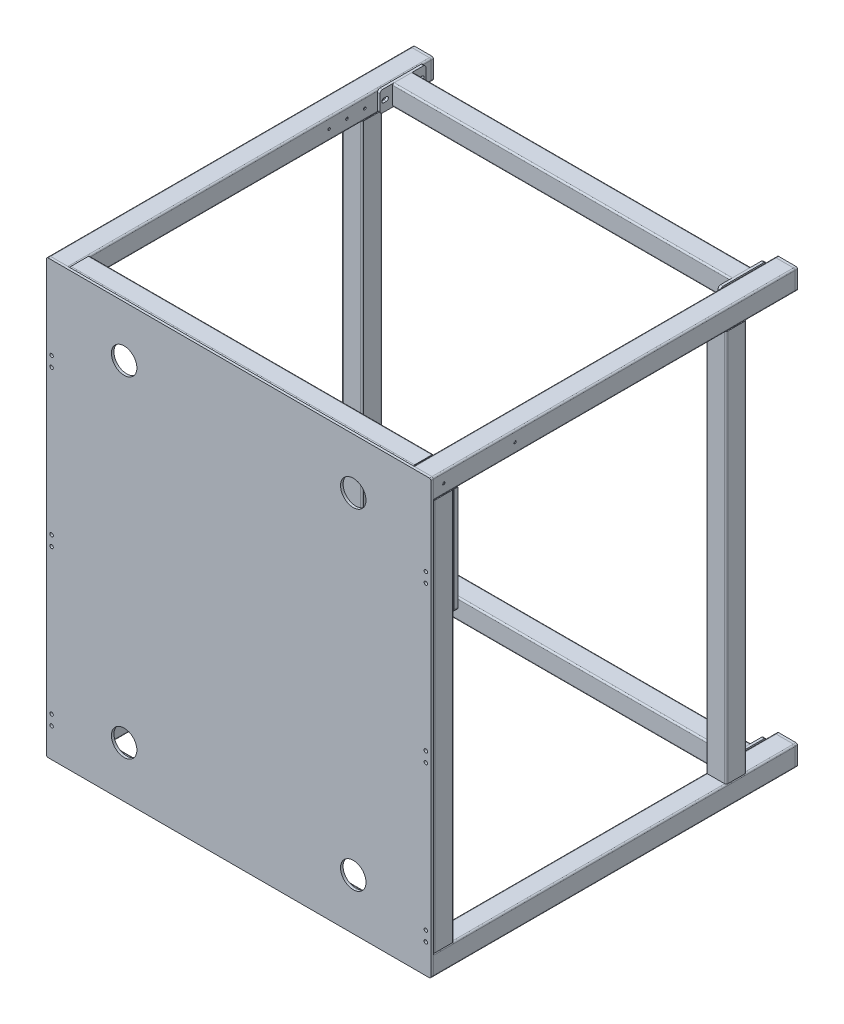
SolidWorks part; units mm, degrees
ref_plane "前视基准面" through (0, 0, 0) normal (0, 0, 1) x (1, 0, 0)
ref_plane "上视基准面" through (0, 0, 0) normal (0, 1, 0) x (1, 0, 0)
ref_plane "右视基准面" through (0, 0, 0) normal (1, 0, 0) x (0, 0, -1)
sketch "草图1" plane through (0, 0, 0) normal (0, 0, 1) x (1, 0, 0)
  line L1 (-377.5, 425) -> (377.5, 425)
  line L2 (-377.5, 425) -> (-377.5, -425)
  line L3 (-377.5, -425) -> (377.5, -425)
  line L4 (377.5, 425) -> (377.5, -425)
  line L5 (-377.5, 425) -> (377.5, -425) construction
  line L6 (-377.5, -425) -> (377.5, 425) construction
  point P0 (0, 0)
  dimension "D1" = 850
  dimension "D2" = 755
extrude "凸台-拉伸1" add sketch "草图1" along normal blind 5
sketch "草图3" plane through (0, 0, 0) normal (0, 0, -1) x (-1, 0, 0)
  line L0 (-377.5, -425) -> (-377.5, 425) construction
  line L1 (-377.5, 425) -> (377.5, 425) construction
  line L2 (377.5, 425) -> (377.5, -425) construction
  line L3 (377.5, -425) -> (-377.5, -425) construction
  line B0 (339.5, 388) -> (339.5, 422)
  line B1 (374.5, 385) -> (340.5, 385)
  line B2 (377.5, 388) -> (377.5, 422)
  line B3 (374.5, 425) -> (340.5, 425)
  line B4 (337.5, 388) -> (337.5, 422)
  line B5 (374.5, 423) -> (340.5, 423)
  line B6 (375.5, 388) -> (375.5, 422)
  line B7 (374.5, 387) -> (340.5, 387)
  arc B8 (377.5, 422) -> (374.5, 425) centre (374.5, 422) ccw
  arc B9 (374.5, 385) -> (377.5, 388) centre (374.5, 388) ccw
  arc B10 (340.5, 385) -> (337.5, 388) centre (340.5, 388) cw
  arc B11 (340.5, 425) -> (337.5, 422) centre (340.5, 422) ccw
  arc B12 (340.5, 423) -> (339.5, 422) centre (340.5, 422) ccw
  arc B13 (375.5, 422) -> (374.5, 423) centre (374.5, 422) ccw
  arc B14 (374.5, 387) -> (375.5, 388) centre (374.5, 388) ccw
  arc B15 (340.5, 387) -> (339.5, 388) centre (340.5, 388) cw
  line B16 (339.5, -422) -> (339.5, -388)
  line B17 (374.5, -425) -> (340.5, -425)
  line B18 (377.5, -422) -> (377.5, -388)
  line B19 (374.5, -385) -> (340.5, -385)
  line B20 (337.5, -422) -> (337.5, -388)
  line B21 (374.5, -387) -> (340.5, -387)
  line B22 (375.5, -422) -> (375.5, -388)
  line B23 (374.5, -423) -> (340.5, -423)
  arc B24 (377.5, -388) -> (374.5, -385) centre (374.5, -388) ccw
  arc B25 (374.5, -425) -> (377.5, -422) centre (374.5, -422) ccw
  arc B26 (340.5, -425) -> (337.5, -422) centre (340.5, -422) cw
  arc B27 (340.5, -385) -> (337.5, -388) centre (340.5, -388) ccw
  arc B28 (340.5, -387) -> (339.5, -388) centre (340.5, -388) ccw
  arc B29 (375.5, -388) -> (374.5, -387) centre (374.5, -388) ccw
  arc B30 (374.5, -423) -> (375.5, -422) centre (374.5, -422) ccw
  arc B31 (340.5, -423) -> (339.5, -422) centre (340.5, -422) cw
  line B32 (-375.5, -422) -> (-375.5, -388)
  line B33 (-340.5, -425) -> (-374.5, -425)
  line B34 (-337.5, -422) -> (-337.5, -388)
  line B35 (-340.5, -385) -> (-374.5, -385)
  line B36 (-377.5, -422) -> (-377.5, -388)
  line B37 (-340.5, -387) -> (-374.5, -387)
  line B38 (-339.5, -422) -> (-339.5, -388)
  line B39 (-340.5, -423) -> (-374.5, -423)
  arc B40 (-337.5, -388) -> (-340.5, -385) centre (-340.5, -388) ccw
  arc B41 (-340.5, -425) -> (-337.5, -422) centre (-340.5, -422) ccw
  arc B42 (-374.5, -425) -> (-377.5, -422) centre (-374.5, -422) cw
  arc B43 (-374.5, -385) -> (-377.5, -388) centre (-374.5, -388) ccw
  arc B44 (-374.5, -387) -> (-375.5, -388) centre (-374.5, -388) ccw
  arc B45 (-339.5, -388) -> (-340.5, -387) centre (-340.5, -388) ccw
  arc B46 (-340.5, -423) -> (-339.5, -422) centre (-340.5, -422) ccw
  arc B47 (-374.5, -423) -> (-375.5, -422) centre (-374.5, -422) cw
  line B48 (-375.5, 388) -> (-375.5, 422)
  line B49 (-340.5, 385) -> (-374.5, 385)
  line B50 (-337.5, 388) -> (-337.5, 422)
  line B51 (-340.5, 425) -> (-374.5, 425)
  line B52 (-377.5, 388) -> (-377.5, 422)
  line B53 (-340.5, 423) -> (-374.5, 423)
  line B54 (-339.5, 388) -> (-339.5, 422)
  line B55 (-340.5, 387) -> (-374.5, 387)
  arc B56 (-337.5, 422) -> (-340.5, 425) centre (-340.5, 422) ccw
  arc B57 (-340.5, 385) -> (-337.5, 388) centre (-340.5, 388) ccw
  arc B58 (-374.5, 385) -> (-377.5, 388) centre (-374.5, 388) cw
  arc B59 (-374.5, 425) -> (-377.5, 422) centre (-374.5, 422) ccw
  arc B60 (-374.5, 423) -> (-375.5, 422) centre (-374.5, 422) ccw
  arc B61 (-339.5, 422) -> (-340.5, 423) centre (-340.5, 422) ccw
  arc B62 (-340.5, 387) -> (-339.5, 388) centre (-340.5, 388) ccw
  arc B63 (-374.5, 387) -> (-375.5, 388) centre (-374.5, 388) cw
sketch_block_instance "方管4040-1"
sketch_block "方管4040" parameters "D2"=3, "D1"=40
sketch_block_instance "方管4040-2"
sketch_block_instance "方管4040-3"
sketch_block_instance "方管4040-4"
extrude "凸台-拉伸3" add sketch "草图3" along normal blind 710 separate body
fillet "圆角1" radius 3 4 edges at (377.5, 425, 2.5) (377.5, -425, 2.5) (-377.5, -425, 2.5) (-377.5, 425, 2.5)
sketch "草图4" plane through (-337.5, 0, 0) normal (1, 0, 0) x (0, 0, -1)
  line L0 (710, -385) -> (0, -385) construction
  line L1 (0, -388) -> (0, -422) construction
  line L2 (0, 422) -> (0, 388) construction
  line L3 (710, 425) -> (0, 425) construction
  line B0 (2, 388) -> (2, 422)
  line B1 (37, 385) -> (3, 385)
  line B2 (40, 388) -> (40, 422)
  line B3 (37, 425) -> (3, 425)
  line B4 (0, 388) -> (0, 422)
  line B5 (37, 423) -> (3, 423)
  line B6 (38, 388) -> (38, 422)
  line B7 (37, 387) -> (3, 387)
  arc B8 (40, 422) -> (37, 425) centre (37, 422) ccw
  arc B9 (37, 385) -> (40, 388) centre (37, 388) ccw
  arc B10 (3, 385) -> (0, 388) centre (3, 388) cw
  arc B11 (3, 425) -> (0, 422) centre (3, 422) ccw
  arc B12 (3, 423) -> (2, 422) centre (3, 422) ccw
  arc B13 (38, 422) -> (37, 423) centre (37, 422) ccw
  arc B14 (37, 387) -> (38, 388) centre (37, 388) ccw
  arc B15 (3, 387) -> (2, 388) centre (3, 388) cw
  line B16 (2, -422) -> (2, -388)
  line B17 (37, -425) -> (3, -425)
  line B18 (40, -422) -> (40, -388)
  line B19 (37, -385) -> (3, -385)
  line B20 (0, -422) -> (0, -388)
  line B21 (37, -387) -> (3, -387)
  line B22 (38, -422) -> (38, -388)
  line B23 (37, -423) -> (3, -423)
  arc B24 (40, -388) -> (37, -385) centre (37, -388) ccw
  arc B25 (37, -425) -> (40, -422) centre (37, -422) ccw
  arc B26 (3, -425) -> (0, -422) centre (3, -422) cw
  arc B27 (3, -385) -> (0, -388) centre (3, -388) ccw
  arc B28 (3, -387) -> (2, -388) centre (3, -388) ccw
  arc B29 (38, -388) -> (37, -387) centre (37, -388) ccw
  arc B30 (37, -423) -> (38, -422) centre (37, -422) ccw
  arc B31 (3, -423) -> (2, -422) centre (3, -422) cw
sketch_block_instance "方管4040-6"
sketch_block_instance "方管4040-8"
extrude "凸台-拉伸4" add sketch "草图4" along normal up to surface (675 mm away) separate body up to face at (337.5, 405, -355)
sketch "草图5" plane through (0, -385, 0) normal (0, 1, 0) x (1, 0, 0)
  line L0 (-377.5, 710) -> (-377.5, 0) construction
  line L1 (-374.5, 0) -> (-340.5, 0) construction
  line L2 (377.5, 710) -> (377.5, 0) construction
  line L3 (340.5, 0) -> (374.5, 0) construction
  line B0 (339.5, 3) -> (339.5, 37)
  line B1 (374.5, 0) -> (340.5, 0)
  line B2 (377.5, 3) -> (377.5, 37)
  line B3 (374.5, 40) -> (340.5, 40)
  line B4 (337.5, 3) -> (337.5, 37)
  line B5 (374.5, 38) -> (340.5, 38)
  line B6 (375.5, 3) -> (375.5, 37)
  line B7 (374.5, 2) -> (340.5, 2)
  arc B8 (377.5, 37) -> (374.5, 40) centre (374.5, 37) ccw
  arc B9 (374.5, 0) -> (377.5, 3) centre (374.5, 3) ccw
  arc B10 (340.5, 0) -> (337.5, 3) centre (340.5, 3) cw
  arc B11 (340.5, 40) -> (337.5, 37) centre (340.5, 37) ccw
  arc B12 (340.5, 38) -> (339.5, 37) centre (340.5, 37) ccw
  arc B13 (375.5, 37) -> (374.5, 38) centre (374.5, 37) ccw
  arc B14 (374.5, 2) -> (375.5, 3) centre (374.5, 3) ccw
  arc B15 (340.5, 2) -> (339.5, 3) centre (340.5, 3) cw
  line B16 (-375.5, 3) -> (-375.5, 37)
  line B17 (-340.5, 0) -> (-374.5, 0)
  line B18 (-337.5, 3) -> (-337.5, 37)
  line B19 (-340.5, 40) -> (-374.5, 40)
  line B20 (-377.5, 3) -> (-377.5, 37)
  line B21 (-340.5, 38) -> (-374.5, 38)
  line B22 (-339.5, 3) -> (-339.5, 37)
  line B23 (-340.5, 2) -> (-374.5, 2)
  arc B24 (-337.5, 37) -> (-340.5, 40) centre (-340.5, 37) ccw
  arc B25 (-340.5, 0) -> (-337.5, 3) centre (-340.5, 3) ccw
  arc B26 (-374.5, 0) -> (-377.5, 3) centre (-374.5, 3) cw
  arc B27 (-374.5, 40) -> (-377.5, 37) centre (-374.5, 37) ccw
  arc B28 (-374.5, 38) -> (-375.5, 37) centre (-374.5, 37) ccw
  arc B29 (-339.5, 37) -> (-340.5, 38) centre (-340.5, 37) ccw
  arc B30 (-340.5, 2) -> (-339.5, 3) centre (-340.5, 3) ccw
  arc B31 (-374.5, 2) -> (-375.5, 3) centre (-374.5, 3) cw
sketch_block_instance "方管4040-10"
sketch_block_instance "方管4040-11"
extrude "凸台-拉伸5" add sketch "草图5" along normal up to surface (770 mm away) separate body up to face at (-357.5, 385, -355)
sketch "草图6" plane through (0, 0, 5) normal (0, 0, 1) x (1, 0, 0)
  line L0 (367.5, 262.5) -> (367.5, -367.5) construction
  line L1 (367.5, 262.5) -> (-367.5, 262.5) construction
  line L2 (367.5, 262.5) -> (367.5, -367.5) construction
  line L3 (367.5, -367.5) -> (-367.5, -367.5) construction
  line L4 (-367.5, 262.5) -> (-367.5, -367.5) construction
  line L5 (367.5, 262.5) -> (-367.5, -367.5) construction
  line L6 (367.5, -367.5) -> (-367.5, 262.5) construction
  line L7 (0, -425) -> (0, -367.5) construction
  line L8 (-374.5, -425) -> (374.5, -425) construction
  circle A0 centre (-367.5, -367.5) radius 3.4
  circle A1 centre (367.5, -367.5) radius 3.4 construction
  circle A2 centre (367.5, 262.5) radius 3.4 construction
  circle A3 centre (-367.5, 262.5) radius 3.4 construction
  circle A4 centre (-367.5, -347.5) radius 3.4
  circle A5 centre (367.5, 262.5) radius 3.4 construction
  circle A6 centre (367.5, 262.5) radius 3.4
  circle A7 centre (-367.5, -62.5) radius 3.4
  circle A8 centre (-367.5, -42.5) radius 3.4
  circle A9 centre (-367.5, 242.5) radius 3.4
  circle A10 centre (-367.5, 262.5) radius 3.4
  circle A11 centre (367.5, 242.5) radius 3.4
  circle A12 centre (367.5, -42.5) radius 3.4
  circle A13 centre (367.5, -62.5) radius 3.4
  circle A14 centre (367.5, -347.5) radius 3.4
  circle A15 centre (367.5, -367.5) radius 3.4
  dimension "D3" = 6.8
  dimension "D5" = 20
  dimension "D6" = 3
  dimension "D1" = 735
  dimension "D2" = 630
  dimension "D4" = 57.5
extrude "切除-拉伸1" cut sketch "草图6" against normal blind 30
sketch "草图7" plane through (0, 0, -710) normal (0, 0, -1) x (-1, 0, 0)
  line L0 (-340.5, 425) -> (-374.5, 425) construction
  line L1 (-377.5, 422) -> (-377.5, 388) construction
  line L2 (377.5, 388) -> (377.5, 422) construction
  line L3 (374.5, 425) -> (340.5, 425) construction
  line L4 (374.5, -385) -> (340.5, -385) construction
  line L5 (377.5, -422) -> (377.5, -388) construction
  line B0 (337.5, 422) -> (337.5, 388)
  line B1 (340.5, 385) -> (374.5, 385)
  line B2 (377.5, 388) -> (377.5, 422)
  line B3 (374.5, 425) -> (340.5, 425)
  circle B4 centre (357.5, 405) radius 9.5
  arc B5 (340.5, 425) -> (337.5, 422) centre (340.5, 422) ccw
  arc B6 (337.5, 388) -> (340.5, 385) centre (340.5, 388) ccw
  arc B7 (374.5, 385) -> (377.5, 388) centre (374.5, 388) ccw
  arc B8 (377.5, 422) -> (374.5, 425) centre (374.5, 422) ccw
  line B9 (337.5, -388) -> (337.5, -422)
  line B10 (340.5, -425) -> (374.5, -425)
  line B11 (377.5, -422) -> (377.5, -388)
  line B12 (374.5, -385) -> (340.5, -385)
  circle B13 centre (357.5, -405) radius 9.5
  arc B14 (340.5, -385) -> (337.5, -388) centre (340.5, -388) ccw
  arc B15 (337.5, -422) -> (340.5, -425) centre (340.5, -422) ccw
  arc B16 (374.5, -425) -> (377.5, -422) centre (374.5, -422) ccw
  arc B17 (377.5, -388) -> (374.5, -385) centre (374.5, -388) ccw
  line B18 (-377.432, -388) -> (-377.432, -422)
  line B19 (-374.432, -425) -> (-340.432, -425)
  line B20 (-337.432, -422) -> (-337.432, -388)
  line B21 (-340.432, -385) -> (-374.432, -385)
  circle B22 centre (-357.432, -405) radius 9.5
  arc B23 (-374.432, -385) -> (-377.432, -388) centre (-374.432, -388) ccw
  arc B24 (-377.432, -422) -> (-374.432, -425) centre (-374.432, -422) ccw
  arc B25 (-340.432, -425) -> (-337.432, -422) centre (-340.432, -422) ccw
  arc B26 (-337.432, -388) -> (-340.432, -385) centre (-340.432, -388) ccw
  line B27 (-377.5, 422) -> (-377.5, 388)
  line B28 (-374.5, 385) -> (-340.5, 385)
  line B29 (-337.5, 388) -> (-337.5, 422)
  line B30 (-340.5, 425) -> (-374.5, 425)
  circle B31 centre (-357.5, 405) radius 9.5
  arc B32 (-374.5, 425) -> (-377.5, 422) centre (-374.5, 422) ccw
  arc B33 (-377.5, 388) -> (-374.5, 385) centre (-374.5, 388) ccw
  arc B34 (-340.5, 385) -> (-337.5, 388) centre (-340.5, 388) ccw
  arc B35 (-337.5, 422) -> (-340.5, 425) centre (-340.5, 422) ccw
sketch_block_instance "方管4040-M16-1"
sketch_block "方管4040-M16" parameters "D1"=19
sketch_block_instance "方管4040-M16-2"
sketch_block_instance "方管4040-M16-3"
sketch_block_instance "方管4040-M16-4"
extrude "凸台-拉伸6" add sketch "草图7" along normal blind 5 separate body
sketch "草图8" plane through (0, 0, -40) normal (0, 0, -1) x (-1, 0, 0)
  line L0 (-377.5, 385) -> (-377.5, -385) construction
  line L1 (-377.5, 175) -> (-317.5, 175)
  line L2 (-377.5, 175) -> (-377.5, 385)
  line L3 (-377.5, 385) -> (-317.5, 385)
  line L4 (-317.5, 175) -> (-317.5, 385)
  line L5 (-374.5, 385) -> (-340.5, 385) construction
  dimension "D1" = 60
  dimension "D2" = 210
extrude "凸台-拉伸7" add sketch "草图8" along normal blind 8 separate body
sketch "草图9" plane through (0, 0, -48) normal (0, 0, -1) x (-1, 0, 0)
  line L0 (-377.5, 280) -> (-317.5, 280) construction
  line L1 (-377.5, 385) -> (-377.5, 175) construction
  line L2 (-317.5, 175) -> (-317.5, 385) construction
  line L4 (-366.5, 187.5) -> (-328.5, 187.5) construction
  line L5 (-366.5, 187.5) -> (-366.5, 352.5) construction
  line L6 (-366.5, 352.5) -> (-328.5, 352.5) construction
  line L7 (-328.5, 187.5) -> (-328.5, 352.5) construction
  line L8 (-366.5, 187.5) -> (-328.5, 352.5) construction
  line L9 (-366.5, 352.5) -> (-328.5, 187.5) construction
  line L10 (-377.5, 175) -> (-317.5, 175) construction
  circle A0 centre (-366.5, 187.5) radius 3.4
  circle A1 centre (-328.5, 187.5) radius 3.4
  circle A2 centre (-366.5, 352.5) radius 3.4
  circle A3 centre (-328.5, 352.5) radius 3.4
  point P6 (-347.5, 270)
  dimension "D3" = 6.8
  dimension "D1" = 165
  dimension "D2" = 11
  dimension "D4" = 12.5
  dimension "D5" = 38
extrude "切除-拉伸2" cut sketch "草图9" against normal blind 10
fillet "圆角2" radius 5 3 edges at (317.5, 385, -44) (317.5, 175, -44) (377.5, 175, -44)
sketch "草图10" plane through (0, 385, 0) normal (0, -1, 0) x (1, 0, 0)
  line L0 (-377.5, -710) -> (-377.5, 0) construction
  line L1 (-340.5, -715) -> (-374.5, -715) construction
  line L2 (337.5, -710) -> (337.5, 0) construction
  line B0 (-375.5, -612) -> (-375.5, -578)
  line B1 (-340.5, -615) -> (-374.5, -615)
  line B2 (-337.5, -612) -> (-337.5, -578)
  line B3 (-340.5, -575) -> (-374.5, -575)
  line B4 (-377.5, -612) -> (-377.5, -578)
  line B5 (-340.5, -577) -> (-374.5, -577)
  line B6 (-339.5, -612) -> (-339.5, -578)
  line B7 (-340.5, -613) -> (-374.5, -613)
  arc B8 (-337.5, -578) -> (-340.5, -575) centre (-340.5, -578) ccw
  arc B9 (-340.5, -615) -> (-337.5, -612) centre (-340.5, -612) ccw
  arc B10 (-374.5, -615) -> (-377.5, -612) centre (-374.5, -612) cw
  arc B11 (-374.5, -575) -> (-377.5, -578) centre (-374.5, -578) ccw
  arc B12 (-374.5, -577) -> (-375.5, -578) centre (-374.5, -578) ccw
  arc B13 (-339.5, -578) -> (-340.5, -577) centre (-340.5, -578) ccw
  arc B14 (-340.5, -613) -> (-339.5, -612) centre (-340.5, -612) ccw
  arc B15 (-374.5, -613) -> (-375.5, -612) centre (-374.5, -612) cw
  line B16 (339.5, -612) -> (339.5, -578)
  line B17 (374.5, -615) -> (340.5, -615)
  line B18 (377.5, -612) -> (377.5, -578)
  line B19 (374.5, -575) -> (340.5, -575)
  line B20 (337.5, -612) -> (337.5, -578)
  line B21 (374.5, -577) -> (340.5, -577)
  line B22 (375.5, -612) -> (375.5, -578)
  line B23 (374.5, -613) -> (340.5, -613)
  arc B24 (377.5, -578) -> (374.5, -575) centre (374.5, -578) ccw
  arc B25 (374.5, -615) -> (377.5, -612) centre (374.5, -612) ccw
  arc B26 (340.5, -615) -> (337.5, -612) centre (340.5, -612) cw
  arc B27 (340.5, -575) -> (337.5, -578) centre (340.5, -578) ccw
  arc B28 (340.5, -577) -> (339.5, -578) centre (340.5, -578) ccw
  arc B29 (375.5, -578) -> (374.5, -577) centre (374.5, -578) ccw
  arc B30 (374.5, -613) -> (375.5, -612) centre (374.5, -612) ccw
  arc B31 (340.5, -613) -> (339.5, -612) centre (340.5, -612) cw
  dimension "D1" = 100
sketch_block_instance "方管4040-14"
sketch_block_instance "方管4040-16"
extrude "凸台-拉伸8" add sketch "草图10" along normal up to surface (770 mm away) separate body up to face at (-357.5, -385, -355)
sketch "草图11" plane through (-337.5, 0, 0) normal (1, 0, 0) x (0, 0, -1)
  line L0 (710, -425) -> (0, -425) construction
  line L1 (605, -425) -> (695, -425)
  line L2 (605, -425) -> (605, -385)
  line L3 (605, -385) -> (695, -385)
  line L4 (695, -425) -> (695, -385)
  line L5 (715, -388) -> (715, -422) construction
  dimension "D1" = 90
  dimension "D2" = 40
  dimension "D3" = 20
extrude "凸台-拉伸9" add sketch "草图11" along normal blind 5 separate body
fillet "圆角3" radius 5 4 edges at (-335, -425, -695) (-335, -385, -695) (-335, -385, -605) (-335, -425, -605)
sketch "草图12" plane through (-332.5, 0, 0) normal (1, 0, 0) x (0, 0, -1)
  line L0 (605, -405) -> (695, -405) construction
  line L1 (605, -390) -> (605, -420) construction
  line L2 (695, -420) -> (695, -390) construction
  line L3 (650, -425) -> (650, -385) construction
  line L4 (610, -425) -> (690, -425) construction
  line L5 (690, -385) -> (610, -385) construction
  line L6 (612.5, -405) -> (617.5, -405) construction
  line L7 (612.5, -401) -> (617.5, -401)
  line L8 (612.5, -409) -> (617.5, -409)
  line L9 (687.5, -405) -> (682.5, -405) construction
  line L10 (687.5, -401) -> (682.5, -401)
  line L11 (687.5, -409) -> (682.5, -409)
  arc A0 (612.5, -401) -> (612.5, -409) centre (612.5, -405) ccw
  arc A1 (617.5, -409) -> (617.5, -401) centre (617.5, -405) ccw
  arc A2 (687.5, -401) -> (687.5, -409) centre (687.5, -405) cw
  arc A3 (682.5, -409) -> (682.5, -401) centre (682.5, -405) cw
  point P14 (615, -405)
  point P21 (685, -405)
  dimension "D1" = 70
  dimension "D2" = 8
  dimension "D3" = 5
extrude "切除-拉伸3" cut sketch "草图12" against normal blind 5
sketch "草图13" plane through (-332.5, 0, 0) normal (1, 0, 0) x (0, 0, -1)
  line L0 (610, -425) -> (690, -425) construction
  line L1 (650, -405) -> (650, -385) construction
  line L2 (690, -385) -> (610, -385) construction
  line B0 (632, -422) -> (632, -388)
  line B1 (667, -425) -> (633, -425)
  line B2 (670, -422) -> (670, -388)
  line B3 (667, -385) -> (633, -385)
  line B4 (630, -422) -> (630, -388)
  line B5 (667, -387) -> (633, -387)
  line B6 (668, -422) -> (668, -388)
  line B7 (667, -423) -> (633, -423)
  arc B8 (670, -388) -> (667, -385) centre (667, -388) ccw
  arc B9 (667, -425) -> (670, -422) centre (667, -422) ccw
  arc B10 (633, -425) -> (630, -422) centre (633, -422) cw
  arc B11 (633, -385) -> (630, -388) centre (633, -388) ccw
  arc B12 (633, -387) -> (632, -388) centre (633, -388) ccw
  arc B13 (668, -388) -> (667, -387) centre (667, -388) ccw
  arc B14 (667, -423) -> (668, -422) centre (667, -422) ccw
  arc B15 (633, -423) -> (632, -422) centre (633, -422) cw
sketch_block_instance "方管4040-18"
extrude "凸台-拉伸10" add sketch "草图13" along normal blind 664 separate body
sketch "草图14" plane through (331.5, 0, 0) normal (1, 0, 0) x (0, 0, -1)
  line L2 (687.5, -401) -> (682.5, -401)
  line L3 (682.5, -409) -> (687.5, -409)
  line L4 (610, -425) -> (690, -425)
  line L5 (695, -420) -> (695, -390)
  line L6 (690, -385) -> (610, -385)
  line L7 (605, -390) -> (605, -420)
  line L8 (610, -425) -> (690, -425)
  line L9 (695, -420) -> (695, -390)
  line L10 (690, -385) -> (610, -385)
  line L11 (605, -390) -> (605, -420)
  line L12 (687.5, -401) -> (682.5, -401)
  line L13 (682.5, -409) -> (687.5, -409)
  line L14 (612.5, -409) -> (617.5, -409)
  line L15 (617.5, -401) -> (612.5, -401)
  line L16 (612.5, -409) -> (617.5, -409)
  line L17 (617.5, -401) -> (612.5, -401)
  arc A2 (682.5, -401) -> (682.5, -409) centre (682.5, -405) ccw
  arc A3 (687.5, -409) -> (687.5, -401) centre (687.5, -405) ccw
  arc A4 (690, -425) -> (695, -420) centre (690, -420) ccw
  arc A5 (695, -390) -> (690, -385) centre (690, -390) ccw
  arc A6 (610, -385) -> (605, -390) centre (610, -390) ccw
  arc A7 (605, -420) -> (610, -425) centre (610, -420) ccw
  arc A8 (690, -425) -> (695, -420) centre (690, -420) ccw
  arc A9 (695, -390) -> (690, -385) centre (690, -390) ccw
  arc A10 (610, -385) -> (605, -390) centre (610, -390) ccw
  arc A11 (605, -420) -> (610, -425) centre (610, -420) ccw
  arc A12 (682.5, -401) -> (682.5, -409) centre (682.5, -405) ccw
  arc A13 (687.5, -409) -> (687.5, -401) centre (687.5, -405) ccw
  arc A14 (617.5, -409) -> (617.5, -401) centre (617.5, -405) ccw
  arc A15 (612.5, -401) -> (612.5, -409) centre (612.5, -405) ccw
  arc A16 (617.5, -409) -> (617.5, -401) centre (617.5, -405) ccw
  arc A17 (612.5, -401) -> (612.5, -409) centre (612.5, -405) ccw
  dimension "D1" = 0
  dimension "D2" = 0
  dimension "D3" = 0
extrude "凸台-拉伸11" add sketch "草图14" along normal blind 5 separate body
sketch "草图15" plane through (-337.5, 0, 0) normal (1, 0, 0) x (0, 0, -1)
  line L0 (710, -385) -> (0, -385) construction
  line L1 (715, -388) -> (715, -422) construction
  line L2 (0, 0) -> (427.9183, 0) construction
  circle A0 centre (685, -405) radius 2.5
  circle A1 centre (650, -405) radius 2.5
  circle A2 centre (615, -405) radius 2.5
  circle A3 centre (580, -405) radius 2.5
  circle A4 centre (545, -405) radius 2.5
  circle A5 centre (510, -405) radius 2.5
  circle A6 centre (510, 405) radius 2.5
  circle A7 centre (545, 405) radius 2.5
  circle A8 centre (580, 405) radius 2.5
  circle A9 centre (615, 405) radius 2.5
  circle A10 centre (650, 405) radius 2.5
  circle A11 centre (685, 405) radius 2.5
  dimension "D2" = 30
  dimension "D3" = 5
  dimension "D1" = 20
  dimension "D4" = 6
extrude "切除-拉伸4" cut sketch "草图15" against normal blind 5 and the other way up to surface
pattern_linear "阵列(线性)1" count 2 spacing 810 along (0, 1, 0) of bodies 132 131 127
sketch "草图16" plane through (0, 0, 5) normal (0, 0, 1) x (1, 0, 0)
  line L0 (0, 0) -> (0, 425) construction
  line L1 (374.5, 425) -> (-374.5, 425) construction
  line L2 (0, 0) -> (225, 0) construction
  circle A0 centre (-225, 325) radius 25
  circle A1 centre (225, 325) radius 25
  circle A2 centre (225, -325) radius 25
  circle A3 centre (-225, -325) radius 25
  dimension "D1" = 50
  dimension "D3" = 100
  dimension "D2" = 450
extrude "切除-拉伸5" cut sketch "草图16" against normal blind 10
sketch "草图17" plane through (377.5, 0, 0) normal (1, 0, 0) x (0, 0, -1)
  line L0 (710, 425) -> (0, 425) construction
  line L1 (-5, -422) -> (-5, 422) construction
  line L2 (20, 405) -> (160, 405) construction
  circle A0 centre (20, 405) radius 2.5
  circle A1 centre (160, 405) radius 2.5
  dimension "D1" = 20
  dimension "D3" = 5
  dimension "D4" = 140
  dimension "D2" = 25
extrude "切除-拉伸6" cut sketch "草图17" against normal blind 1.5
